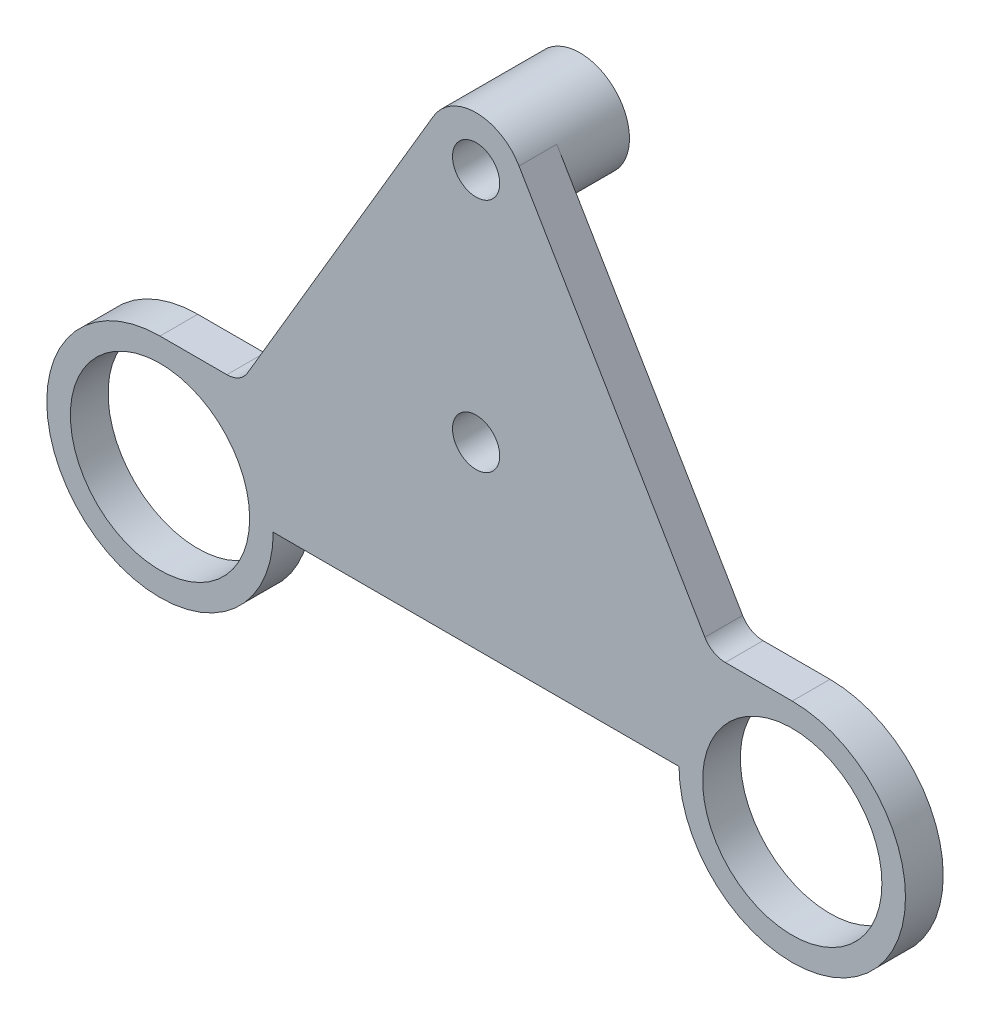
SolidWorks part; units mm, degrees
ref_plane "前视基准面" through (0, 0, 0) normal (0, 0, 1) x (1, 0, 0)
ref_plane "上视基准面" through (0, 0, 0) normal (0, 1, 0) x (1, 0, 0)
ref_plane "右视基准面" through (0, 0, 0) normal (1, 0, 0) x (0, 0, -1)
other "Configuration Table"
sketch "草图1" plane through (0, 0, 0) normal (0, 0, 1) x (1, 0, 0)
  line L0 (0, 0) -> (0, 38) construction
  line L1 (-43, 0) -> (-122.0563, 0) construction
  line L2 (0, 0) -> (0, -34.5403) construction
  line L3 (-67, 36.5806) -> (-67, -34.5403) construction
  line L4 (-43, 0) -> (43, 0)
  line L5 (43, 0) -> (122.0563, 0) construction
  line L6 (67, 36.5806) -> (67, -34.5403) construction
  line L7 (-122.0563, 88) -> (130.5675, 88) construction
  line L8 (-43, 38) -> (-5, 38) construction
  line L9 (-67, 24) -> (-52.7845, 24)
  line L10 (-52.7845, 24) -> (-52.7845, 29) construction
  line L13 (67, 24) -> (52.7845, 24)
  line L14 (-9.0933, 93.25) -> (-48.4775, 26.4602)
  line L15 (9.0933, 93.25) -> (48.4775, 26.4602)
  line L16 (0, 38) -> (43, 38) construction
  line L17 (0, 88) -> (0, 341.9814) construction
  circle A0 centre (-67, 0) radius 19
  arc A1 (-67, 24) -> (-43, 0) centre (-67, 0) ccw
  arc A2 (67, 24) -> (43, 0) centre (67, 0) cw
  circle A3 centre (67, 0) radius 19
  arc A5 (9.0933, 93.25) -> (-9.0933, 93.25) centre (0, 88) ccw
  arc A6 (-52.8201, 24) -> (-48.4775, 26.4602) centre (-52.7845, 29) ccw
  arc A7 (52.8201, 24) -> (48.4775, 26.4602) centre (52.7845, 29) cw
  circle A8 centre (0, 88) radius 5
  circle A9 centre (0, 38) radius 5
  dimension "D2" = 88
  dimension "D4" = 14.2155
  dimension "D6" = 10.5
  dimension "D1" = 67
  dimension "D3" = 38
extrude "凸台-拉伸1" add sketch "草图1" along normal blind 8 contours L13 A7 L15 A5 L14 A6 L9 A1 L4 A2 A3 A0
sketch "草图3" plane through (0, 0, 0) normal (0, 0, -1) x (-1, 0, 0)
  line L0 (0, 0) -> (0, 76) construction
  line L1 (-9.0933, 93.25) -> (0, 88) construction
  circle A0 centre (0, 88) radius 10.5
  circle A1 centre (0, 38) radius 10.5
  circle A2 centre (0, 88) radius 5
  circle A3 centre (0, 38) radius 5
  dimension "D1" = 50
extrude "凸台-拉伸3" add sketch "草图3" along normal blind 14
sketch "草图6" plane through (0, 0, -14) normal (0, 0, -1) x (-1, 0, 0)
